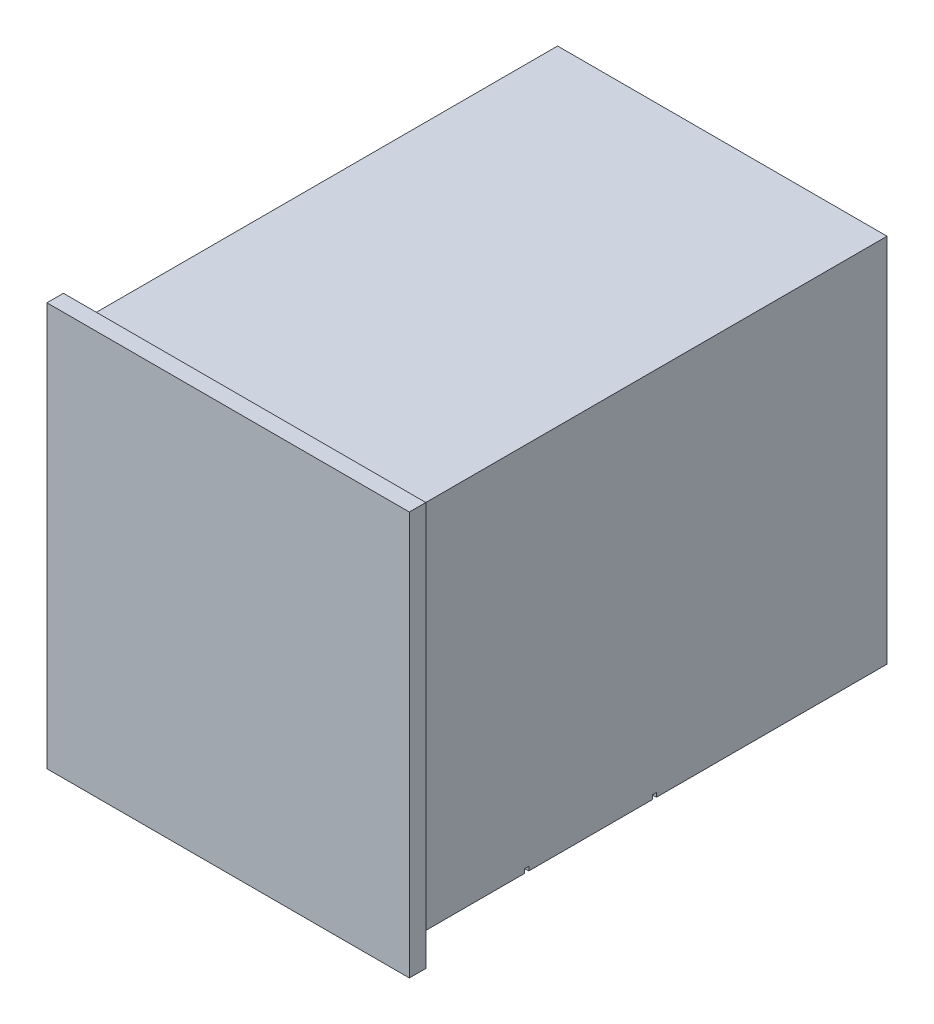
SolidWorks part; units mm, degrees
material "ABS"
ref_plane "Front Plane" through (0, 0, 0) normal (0, 0, 1) x (1, 0, 0)
ref_plane "Top Plane" through (0, 0, 0) normal (0, 1, 0) x (1, 0, 0)
ref_plane "Right Plane" through (0, 0, 0) normal (1, 0, 0) x (0, 0, -1)
sketch "Sketch1" plane through (0, 0, 0) normal (0, 0, 1) x (1, 0, 0)
  line L1 (0, 0) -> (400, 0)
  line L2 (0, 0) -> (0, 450)
  line L3 (0, 450) -> (400, 450)
  line L4 (400, 0) -> (400, 450)
  dimension "D1" = 450
  dimension "D2" = 400
extrude "Boss-Extrude1" add sketch "Sketch1" along normal blind 600
sketch "Sketch2" plane through (0, 0, 600) normal (0, 0, 1) x (1, 0, 0)
  line L0 (400, 450) -> (0, 450) construction
  line L1 (-20, 470) -> (420, 470)
  line L2 (-20, 470) -> (-20, -20)
  line L3 (-20, -20) -> (420, -20)
  line L4 (420, 470) -> (420, -20)
  line L5 (400, 0) -> (400, 450) construction
  line L6 (0, 450) -> (0, 0) construction
  line L7 (0, 0) -> (400, 0) construction
  dimension "D1" = 20
  dimension "D2" = 20
  dimension "D3" = 20
  dimension "D4" = 20
extrude "Boss-Extrude2" add sketch "Sketch2" against normal blind 20
sketch "Sketch3" plane through (0, 0, 0) normal (0, -1, 0) x (1, 0, 0)
  line L0 (0, 580) -> (0, 0) construction
  line L1 (0, 440) -> (400, 440)
  line L2 (0, 440) -> (0, 435)
  line L3 (0, 435) -> (400, 435)
  line L4 (400, 440) -> (400, 435)
  line L5 (400, 580) -> (400, 0) construction
  line L6 (0, 580) -> (400, 580) construction
  dimension "D1" = 140
  dimension "D2" = 5
extrude "Cut-Extrude1" cut sketch "Sketch3" against normal blind 5
sketch "Sketch4" plane through (0, 0, 0) normal (0, -1, 0) x (1, 0, 0)
  line L0 (0, 435) -> (0, 0) construction
  line L1 (0, 285) -> (400, 285)
  line L2 (0, 285) -> (0, 280)
  line L3 (0, 280) -> (400, 280)
  line L4 (400, 285) -> (400, 280)
  line L5 (400, 435) -> (400, 0) construction
  line L6 (0, 435) -> (400, 435) construction
  dimension "D1" = 5
  dimension "D2" = 150
extrude "Cut-Extrude2" cut sketch "Sketch4" against normal blind 5
sketch "Sketch5" plane through (0, 0, 0) normal (0, -1, 0) x (1, 0, 0)
  line L0 (0, 580) -> (400, 580) construction
  line L1 (150, 515) -> (250, 515)
  line L2 (150, 515) -> (150, 505)
  line L3 (150, 505) -> (250, 505)
  line L4 (250, 515) -> (250, 505)
  line L5 (400, 440) -> (0, 440) construction
  line L6 (0, 580) -> (0, 440) construction
  line L7 (400, 580) -> (400, 440) construction
  point P10 (400, 510)
  dimension "D1" = 65
  dimension "D2" = 65
  dimension "D3" = 150
  dimension "D4" = 150
extrude "Boss-Extrude3" add sketch "Sketch5" along normal blind 20
sketch "Sketch6" plane through (0, 0, 0) normal (0, -1, 0) x (1, 0, 0)
  line L0 (0, 435) -> (400, 435) construction
  line L1 (150, 365) -> (250, 365)
  line L2 (150, 365) -> (150, 355)
  line L3 (150, 355) -> (250, 355)
  line L4 (250, 365) -> (250, 355)
  line L5 (400, 285) -> (0, 285) construction
  line L6 (400, 435) -> (400, 285) construction
  line L7 (0, 435) -> (0, 285) construction
  dimension "D1" = 70
  dimension "D2" = 70
  dimension "D3" = 150
  dimension "D4" = 150
extrude "Boss-Extrude4" add sketch "Sketch6" along normal blind 20
sketch "Sketch7" plane through (0, 0, 0) normal (0, -1, 0) x (1, 0, 0)
  line L0 (0, 280) -> (400, 280) construction
  line L1 (150, 150) -> (250, 150)
  line L2 (150, 150) -> (150, 160)
  line L3 (150, 160) -> (250, 160)
  line L4 (250, 150) -> (250, 160)
  dimension "D1" = 120
  dimension "D2" = 10
extrude "Boss-Extrude5" add sketch "Sketch7" along normal blind 20
sketch "Sketch8" plane through (0, 0, 515) normal (0, 0, 1) x (1, 0, 0)
  line L0 (250, -20) -> (150, -20) construction
  line L1 (155, -0.3339) -> (245, -0.3339)
  line L2 (155, -0.3339) -> (155, -15)
  line L3 (155, -15) -> (245, -15)
  line L4 (245, -0.3339) -> (245, -15)
  line L5 (150, -20) -> (150, 0) construction
  line L6 (250, -20) -> (250, 0) construction
  dimension "D1" = 5
  dimension "D2" = 5
  dimension "D3" = 5
extrude "Cut-Extrude3" cut sketch "Sketch8" against normal blind 500
